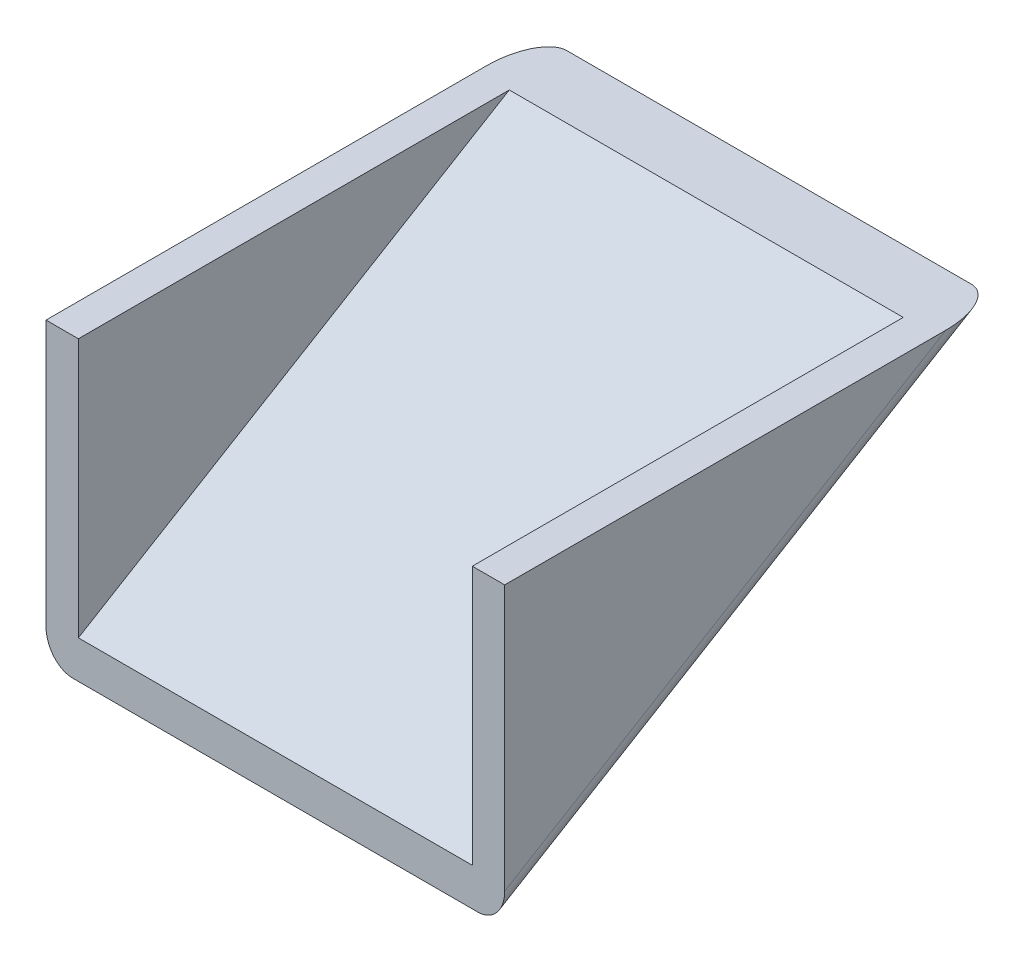
SolidWorks part; units mm, degrees
material "1023 碳钢板 (SS)"
ref_plane "前视基准面" through (0, 0, 0) normal (0, 0, 1) x (1, 0, 0)
ref_plane "上视基准面" through (0, 0, 0) normal (0, 1, 0) x (1, 0, 0)
ref_plane "右视基准面" through (0, 0, 0) normal (1, 0, 0) x (0, 0, -1)
sketch "草图2" plane through (0, 0, 0) normal (0, 0, 1) x (1, 0, 0)
  line L1 (85, 55) -> (-85, 55)
  line L2 (85, 55) -> (85, -55)
  line L3 (85, -55) -> (-85, -55)
  line L4 (-85, 55) -> (-85, -55)
  line L5 (85, 55) -> (-85, -55) construction
  line L6 (85, -55) -> (-85, 55) construction
  point P0 (0, 0)
  dimension "D1" = 170
  dimension "D2" = 110
extrude "凸台-拉伸2" add sketch "草图2" along normal blind 500 contours L2 L1 L4 L3
sketch "草图5" plane through (-85, 0, 0) normal (-1, 0, 0) x (0, 0, 1)
  line L0 (386.9483, 55) -> (386.9483, -55)
  line L1 (500, 55) -> (0, 55) construction
  line L2 (500, -55) -> (0, -55) construction
  line L3 (386.9483, -55) -> (203.9483, 55)
  line L4 (203.9483, 55) -> (386.9483, 55)
  dimension "D1" = 183
extrude "切除-拉伸3" cut sketch "草图5" against normal blind 200 flip side to cut
fillet "圆角2" radius 10 2 edges at (85, 0, 295.4483) (-85, 0, 295.4483)
shell "抽壳2" thickness 12
